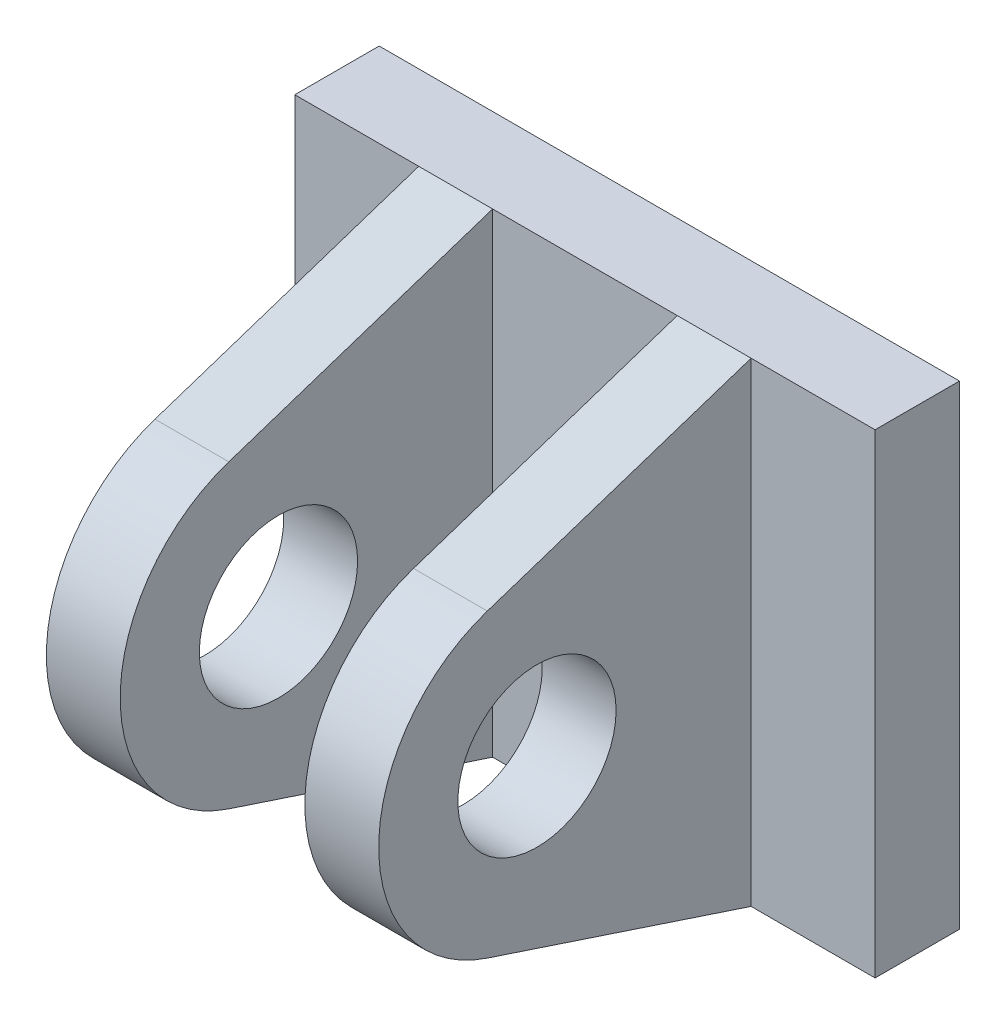
SolidWorks part; units mm, degrees
ref_plane "前视基准面" through (0, 0, 0) normal (0, 0, 1) x (1, 0, 0)
ref_plane "上视基准面" through (0, 0, 0) normal (0, 1, 0) x (1, 0, 0)
ref_plane "右视基准面" through (0, 0, 0) normal (1, 0, 0) x (0, 0, -1)
other "Configuration Table"
sketch "草图1" plane through (0, 0, 0) normal (0, 0, 1) x (1, 0, 0)
  line L1 (-55, -45) -> (55, -45)
  line L2 (-55, -45) -> (-55, 45)
  line L3 (-55, 45) -> (55, 45)
  line L4 (55, -45) -> (55, 45)
  line L5 (0, 45) -> (0, -45) construction
  line L6 (-55, 0) -> (55, 0) construction
  point P0 (0, 0)
  dimension "D1" = 110
  dimension "D2" = 90
extrude "凸台-拉伸1" add sketch "草图1" along normal blind 16
ref_plane "基准面1" through (17.5, 0, 0) normal (1, 0, 0) x (0, 0, -1)
sketch "草图2" plane through (17.5, 0, 0) normal (1, 0, 0) x (0, 0, -1)
  line L0 (-16, 45) -> (-66, 28.4866)
  line L1 (-16, -45) -> (-66, -28.4866)
  line L3 (0, 0) -> (-56.5918, 0) construction
  line L8 (0, -45) -> (0, 45)
  line L9 (0, 45) -> (-16, 45)
  line L10 (-16, 45) -> (-16, -45)
  line L11 (-16, -45) -> (0, -45)
  line L14 (-16, 45) -> (-16, -45)
  arc A0 (-66, -28.4866) -> (-66, 28.4866) centre (-56.5918, 0) cw
  dimension "D2" = 30
  dimension "D1" = 50
  dimension "D3" = 50
  dimension "D4" = 0
extrude "凸台-拉伸2" add sketch "草图2" along normal blind 14 separate body
sketch "草图3" plane through (31.5, 0, 0) normal (1, 0, 0) x (0, 0, -1)
  circle A0 centre (-56.5918, 0) radius 15
  dimension "D1" = 30
extrude "切除-拉伸1" cut sketch "草图3" against normal up to next (14 mm away)
mirror "镜向1" about plane through (0, 0, 0) normal (1, 0, 0) of bodies 108
